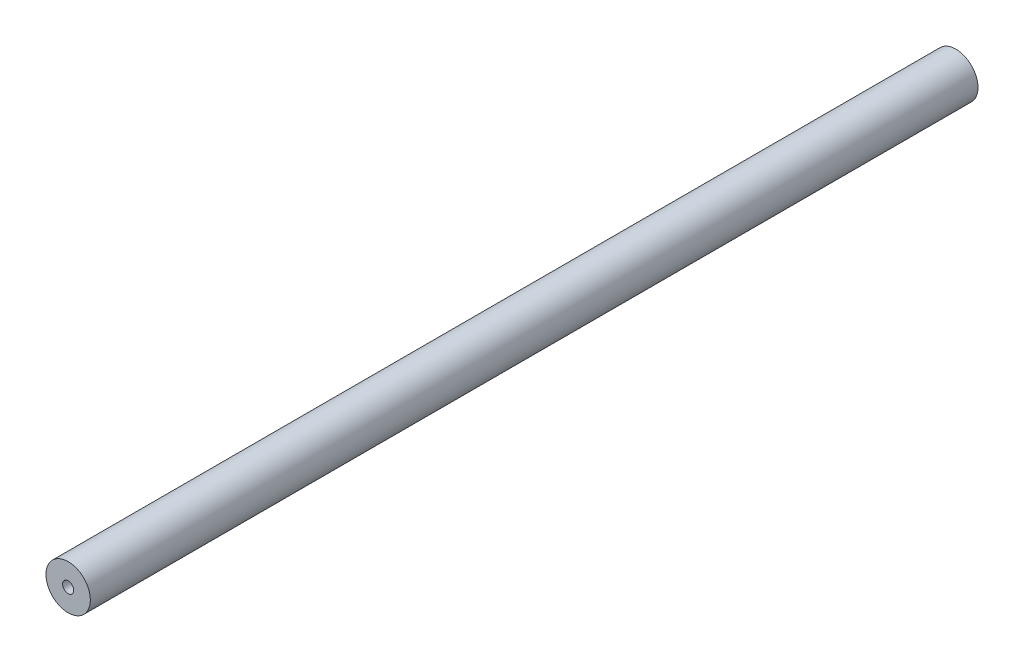
from build123d import *

# Parameters (mm, degrees)
SKETCH1_R             = 10
BOSS_EXTRUDE1_DEPTH   = 400
M6_TAPPED_HOLE1_D     = 5
M6_TAPPED_HOLE1_DEPTH = 15
M6_TAPPED_HOLE1_TIP   = 1.502151548
M6_TAPPED_HOLE2_D     = 5
M6_TAPPED_HOLE2_DEPTH = 15
M6_TAPPED_HOLE2_TIP   = 1.502151548


with BuildPart() as part:
    # Sketch1 → Boss-Extrude1 (new body)
    with BuildSketch(Plane.XY):
        Circle(SKETCH1_R)
    extrude(amount=BOSS_EXTRUDE1_DEPTH)

    # M6 Tapped Hole1
    with Locations(Plane.XY.offset(400)):
        with Locations((0, 0)):
            Hole(M6_TAPPED_HOLE1_D / 2, depth=M6_TAPPED_HOLE1_DEPTH)
            with Locations((0, 0, -(M6_TAPPED_HOLE1_DEPTH + M6_TAPPED_HOLE1_TIP / 2))):  # 118° drill point
                Cone(0, M6_TAPPED_HOLE1_D / 2, M6_TAPPED_HOLE1_TIP, mode=Mode.SUBTRACT)

    # M6 Tapped Hole2
    with Locations(Plane(origin=(0, 0, 0), x_dir=(-1, 0, 0), z_dir=(0, 0, -1))):
        with Locations((0, 0)):
            Hole(M6_TAPPED_HOLE2_D / 2, depth=M6_TAPPED_HOLE2_DEPTH)
            with Locations((0, 0, -(M6_TAPPED_HOLE2_DEPTH + M6_TAPPED_HOLE2_TIP / 2))):  # 118° drill point
                Cone(0, M6_TAPPED_HOLE2_D / 2, M6_TAPPED_HOLE2_TIP, mode=Mode.SUBTRACT)


solid = part.part
